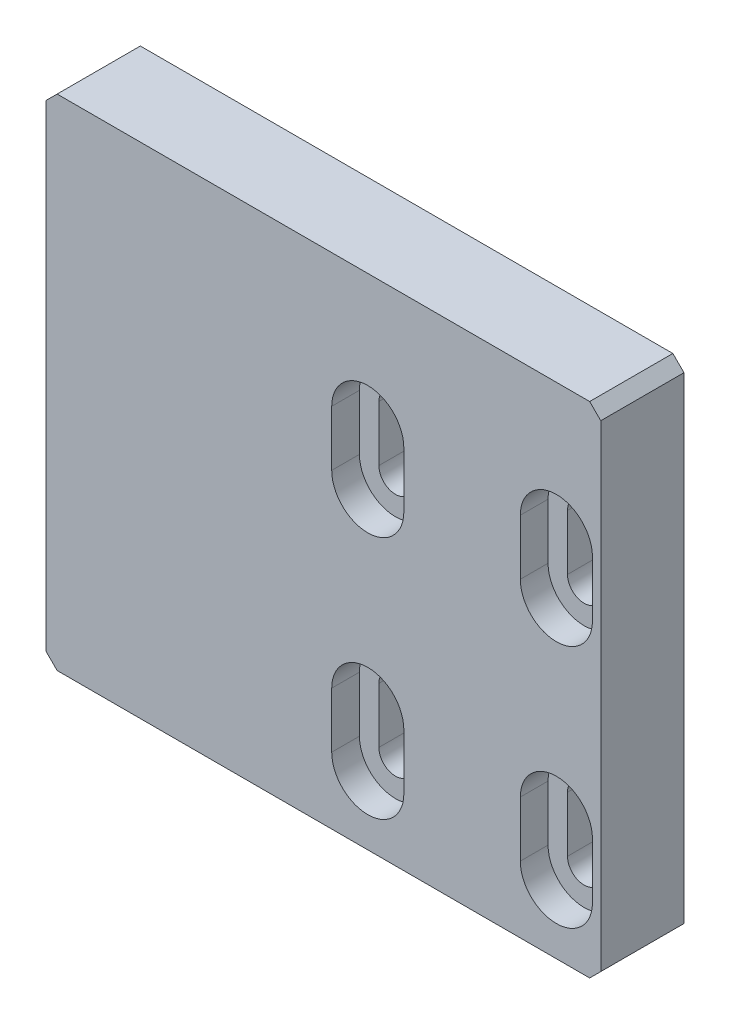
from build123d import *

# Parameters (mm, degrees)
SKETCH_1_W                  = 100
SKETCH_1_H                  = 90
EXTRUDE_1_DEPTH             = 7.5
HOLE_WIZARD_M6_1_D          = 5
HOLE_WIZARD_M6_1_DEPTH      = 15
HOLE_WIZARD_M6_1_TIP        = 1.502151548
CUT_EXTRUDE_1_DEPTH         = 5
CUT_EXTRUDE_2_DEPTH         = 69.007352544
PATTERN_LINEAR_1_COUNT      = 2
PATTERN_LINEAR_1_PITCH      = 34
PATTERN_LINEAR_1_COUNT_DIR2 = 2
PATTERN_LINEAR_1_PITCH_DIR2 = 44
CHAMFER_1_SIZE              = 2


with BuildPart() as part:
    # 草图1 → 凸台-拉伸1 (new, symmetric)
    with BuildSketch(Plane.XY):
        Rectangle(SKETCH_1_W, SKETCH_1_H)
    extrude(amount=EXTRUDE_1_DEPTH, both=True)

    # M6 螺纹孔1
    with Locations(Plane.ZY.offset(50)):
        with Locations((0, 35), (0, 0), (0, -35)):
            Hole(HOLE_WIZARD_M6_1_D / 2, depth=HOLE_WIZARD_M6_1_DEPTH)
            with Locations((0, 0, -(HOLE_WIZARD_M6_1_DEPTH + HOLE_WIZARD_M6_1_TIP / 2))):  # 118° drill point
                Cone(0, HOLE_WIZARD_M6_1_D / 2, HOLE_WIZARD_M6_1_TIP, mode=Mode.SUBTRACT)

    # 草图4 → 切除-拉伸1 (cut)
    with BuildSketch(Plane.XY.offset(7.5)):
        with BuildLine():
            Line((14.5, -23), (14.5, -33))
            ThreePointArc((14.5, -33), (8, -39.5), (1.5, -33))
            Line((1.5, -33), (1.5, -23))
            ThreePointArc((1.5, -23), (8, -16.5), (14.5, -23))
        make_face()
    cut_extrude_1 = extrude(amount=-CUT_EXTRUDE_1_DEPTH, mode=Mode.SUBTRACT)

    # 草图5 → 切除-拉伸2 (cut, through all)
    with BuildSketch(Plane.XY.offset(2.5)):
        with BuildLine():
            Line((5, -23), (5, -33))
            ThreePointArc((5, -33), (8, -36), (11, -33))
            Line((11, -33), (11, -23))
            ThreePointArc((11, -23), (8, -20), (5, -23))
        make_face()
    cut_extrude_2 = extrude(amount=-CUT_EXTRUDE_2_DEPTH, mode=Mode.SUBTRACT)

    # 阵列(线性)1: 切除-拉伸1, Cut-Extrude 2 2 × 2
    with Locations(*[(i * PATTERN_LINEAR_1_PITCH, j * PATTERN_LINEAR_1_PITCH_DIR2, 0) for i in range(PATTERN_LINEAR_1_COUNT) for j in range(PATTERN_LINEAR_1_COUNT_DIR2) if (i, j) != (0, 0)]):
        add(cut_extrude_1, mode=Mode.SUBTRACT)
        add(cut_extrude_2, mode=Mode.SUBTRACT)

    # 倒角1
    chamfer_1_edges = [part.edges().sort_by_distance(p)[0] for p in [
        (50, -45, 0),
        (-50, -45, 0),
        (-50, 45, 0),
        (50, 45, 0),
    ]]
    chamfer(chamfer_1_edges, length=CHAMFER_1_SIZE)


solid = part.part
